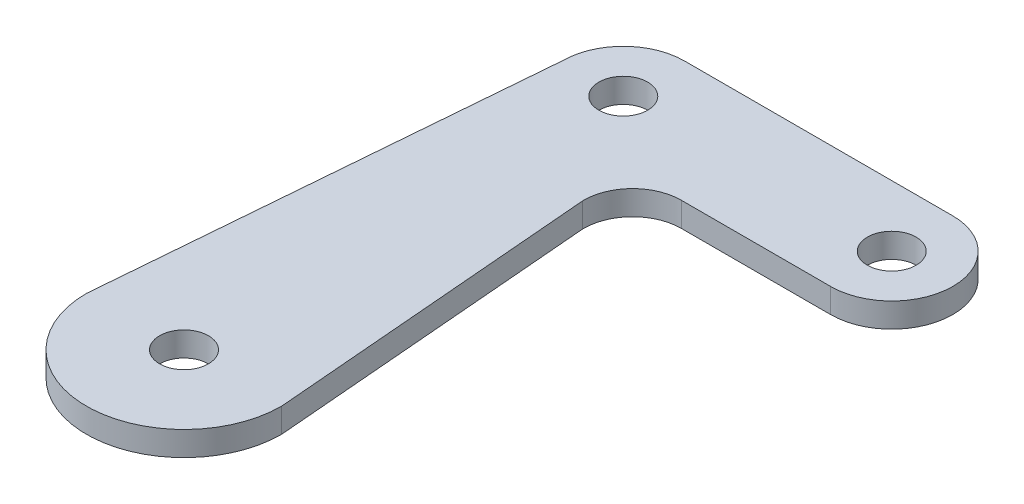
SolidWorks part; units mm, degrees
ref_plane "Front Plane" through (0, 0, 0) normal (0, 0, 1) x (1, 0, 0)
ref_plane "Top Plane" through (0, 0, 0) normal (0, 1, 0) x (1, 0, 0)
ref_plane "Right Plane" through (0, 0, 0) normal (1, 0, 0) x (0, 0, -1)
sketch "Sketch1" plane through (0, 0, 0) normal (0, 1, 0) x (1, 0, 0)
  line L0 (0, 0) -> (0, 77.4861) construction
  line L1 (0, 0) -> (0, -118.7322) construction
  line L2 (0, 0) -> (94.9248, 0) construction
  line L3 (0, 0) -> (-94.903, 0) construction
  line L4 (0, -57.15) -> (-52.6318, -57.15) construction
  line L5 (0, -57.15) -> (36.2897, -57.15) construction
  line L6 (34.925, 0) -> (34.925, -29.4401) construction
  line L7 (34.925, 0) -> (34.925, 20.6268) construction
  line L8 (-12.7, -57.15) -> (12.7, -57.15)
  line L9 (0, 7.9502) -> (34.925, 7.9502)
  line L10 (-7.9502, 0) -> (-12.7, -57.15)
  line L11 (34.925, -7.9502) -> (15.4979, -7.9502)
  line L12 (12.7, -57.15) -> (9.1491, -14.4258)
  circle A0 centre (34.925, 0) radius 3.175
  circle A1 centre (0, 0) radius 3.175
  circle A2 centre (0, -57.15) radius 3.175
  arc A7 (-12.7, -57.15) -> (12.7, -57.15) centre (0, -57.15) ccw
  arc A8 (0, 7.9502) -> (-7.9502, 0) centre (0, 0) ccw
  arc A9 (34.925, 7.9502) -> (34.925, -7.9502) centre (34.925, 0) cw
  arc A10 (15.4979, -7.9502) -> (9.1491, -14.4258) centre (15.4979, -14.3002) ccw
  point P5 (34.925, 0)
  point P22 (24.6018, -7.9502)
  point P25 (11.3364, -14.3002)
  dimension "D2" = 6.35
  dimension "D3" = 6.35
  dimension "D4" = 6.35
  dimension "D5" = 7.9502
  dimension "D6" = 7.9502
  dimension "D8" = 6.35
  dimension "D9" = 12.7
  dimension "D1" = 34.925
  dimension "D7" = 57.15
extrude "Boss-Extrude1" add sketch "Sketch1" along normal blind 3.175 contours A10 L11 A9 L9 A8 L10 L8 A2 L12 A1 A0 | L8 A7 A2
